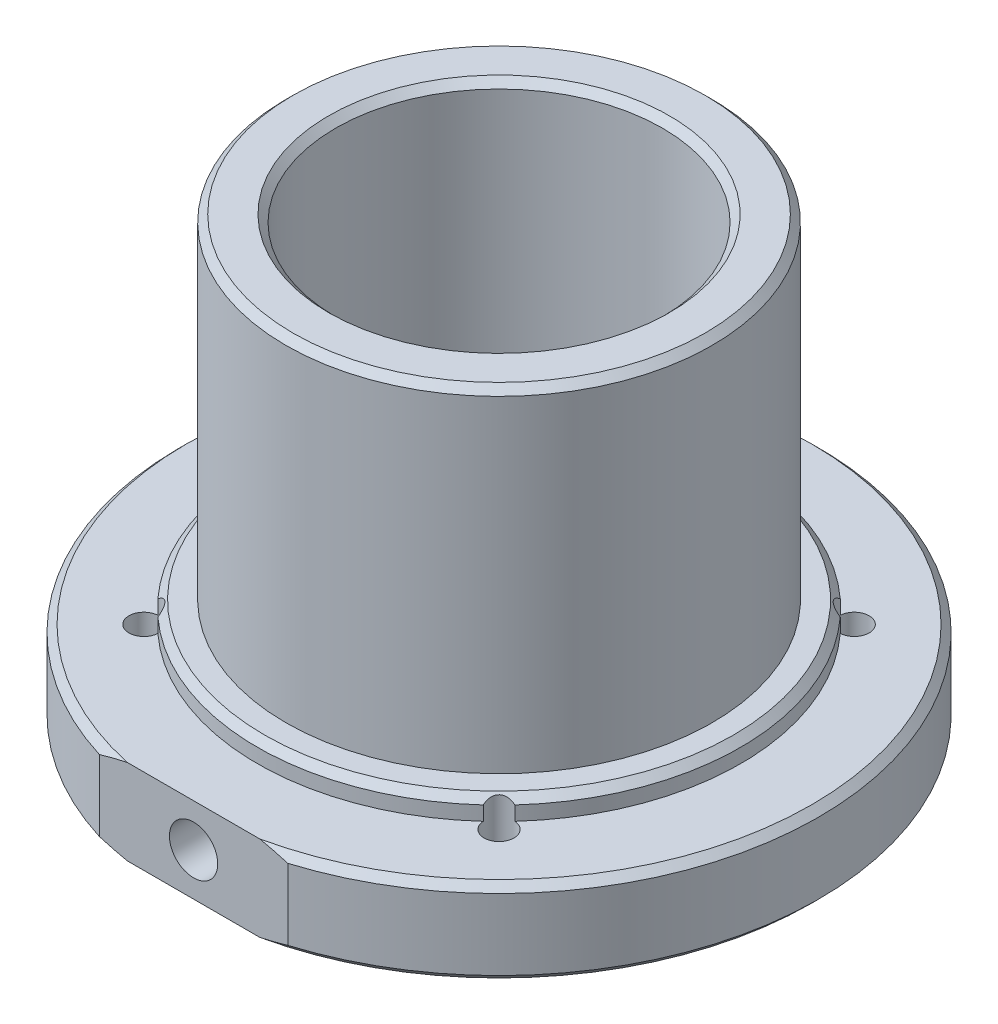
from build123d import *

# Parameters (mm, degrees)
SKETCH_1_R              = 45
EXTRUDE_1_DEPTH         = 12
SKETCH_2_R              = 30
EXTRUDE_2_DEPTH         = 50
SKETCH_11_R             = 34
EXTRUDE_3_DEPTH         = 3
SKETCH_3_R              = 23
CUT_EXTRUDE_1_DEPTH     = 89.848185125
CHAMFER_1_SIZE          = 1
HOLE_WIZARD_M5_1_D      = 4.2
CUT_EXTRUDE_2_DEPTH     = 89.848185125
HOLE_WIZARD_M8_1_REACH  = 118.675
HOLE_WIZARD_M8_1_BORE_R = 3.4


with BuildPart() as part:
    # 草图1 → 凸台-拉伸1 (new body)
    with BuildSketch(Plane(origin=(0, 0, 0), x_dir=(1, 0, 0), z_dir=(0, 1, 0))):
        with Locations(Location((0, 0, 0), (0, 0, 270))):
            Circle(SKETCH_1_R)
    extrude(amount=EXTRUDE_1_DEPTH)

    # 草图2 → 凸台-拉伸2 (add)
    with BuildSketch(Plane(origin=(0, 12, 0), x_dir=(1, 0, 0), z_dir=(0, 1, 0))):
        with Locations(Location((0, 0, 0), (0, 0, 270))):
            Circle(SKETCH_2_R)
    extrude(amount=EXTRUDE_2_DEPTH)

    # 草图11 → 凸台-拉伸3 (add)
    with BuildSketch(Plane(origin=(0, 12, 0), x_dir=(1, 0, 0), z_dir=(0, 1, 0))):
        with Locations(Location((0, 0, 0), (0, 0, 270))):
            Circle(SKETCH_11_R)
    extrude(amount=EXTRUDE_3_DEPTH)

    # 草图3 → 切除-拉伸1 (cut, through all)
    with BuildSketch(Plane.XZ):
        with Locations(Location((0, 0, 0), (0, 0, 270))):
            Circle(SKETCH_3_R)
    extrude(amount=-CUT_EXTRUDE_1_DEPTH, mode=Mode.SUBTRACT)

    # 倒角1
    chamfer_1_edges = [part.edges().sort_by_distance(p)[0] for p in [
        (0, 15, -34),
        (0, 62, 23),
        (0, 0, 23),
        (0, 0, -45),
        (0, 12, -45),
        (0, 62, -30),
    ]]
    chamfer(chamfer_1_edges, length=CHAMFER_1_SIZE)

    # M5 螺纹孔1 (through all)
    with Locations(Plane(origin=(0, 0, 0), x_dir=(-1, 0, 0), z_dir=(0, -1, 0))):
        with Locations((25, -25), (-25, -25), (-25, 25), (25, 25)):
            Hole(HOLE_WIZARD_M5_1_D / 2)

    # 草图8 → 切除-拉伸2 (cut, through all)
    with BuildSketch(Plane.XZ):
        with BuildLine():
            Line((-13.266499161, 43), (13.266499161, 43))
            ThreePointArc((13.266499161, 43), (0, 45), (-13.266499161, 43))
        make_face()
    extrude(amount=-CUT_EXTRUDE_2_DEPTH, mode=Mode.SUBTRACT)

    # M8 螺纹孔1 bore → M8 螺纹孔1 (cut, up to next)
    with BuildSketch(Plane.XY.offset(43), mode=Mode.PRIVATE) as hole_wizard_m8_1_sk1:
        with Locations((0, 6)):
            Circle(HOLE_WIZARD_M8_1_BORE_R)
    hole_wizard_m8_1_tool1 = extrude(hole_wizard_m8_1_sk1.sketch, amount=-HOLE_WIZARD_M8_1_REACH, mode=Mode.PRIVATE) & part.part
    add(hole_wizard_m8_1_tool1.solids().sort_by_distance((0, 6, 43))[0], mode=Mode.SUBTRACT)


solid = part.part
